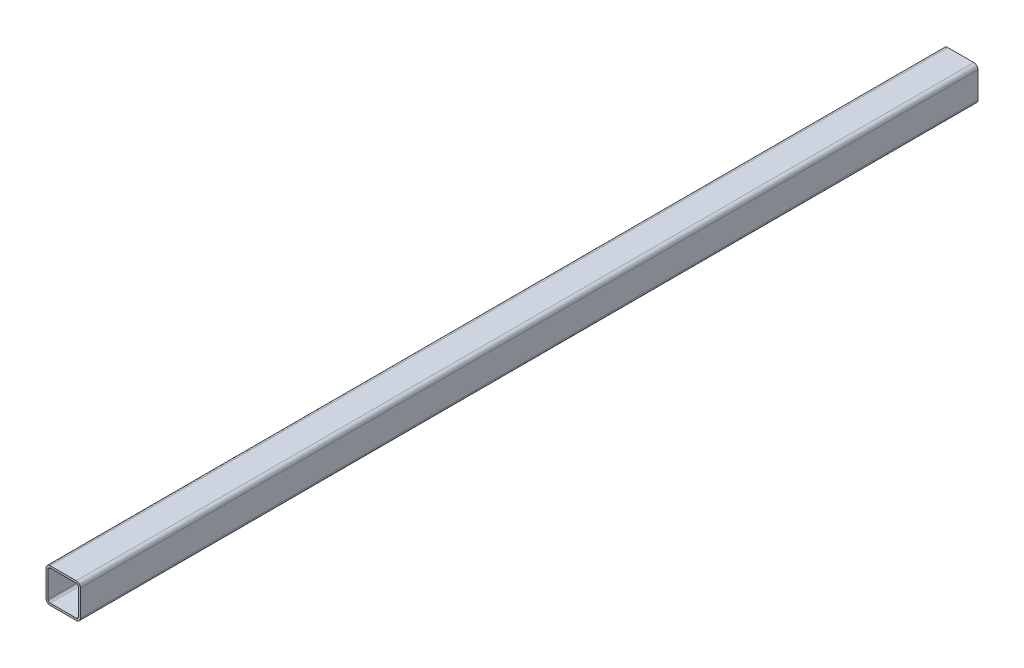
SolidWorks part; units mm, degrees
material "Q235B"
ref_plane "前视基准面" through (0, 0, 0) normal (0, 0, 1) x (1, 0, 0)
ref_plane "上视基准面" through (0, 0, 0) normal (0, 1, 0) x (1, 0, 0)
ref_plane "右视基准面" through (0, 0, 0) normal (1, 0, 0) x (0, 0, -1)
other "Configuration Table"
sketch "草图1" plane through (0, 0, 0) normal (1, 0, 0) x (0, 0, -1)
  line L0 (-652.5, 0) -> (652.5, 0)
other "Gb／6728-1986方形空心型钢 050 X 50 X 3(1)"
ref_plane "基准面1" through (0, 0, 652.5) normal (0, 0, -1) x (0, 1, 0)
sketch "Sketch1" plane through (0, 0, 652.5) normal (0, 0, -1) x (0, 1, 0)
  line L0 (-19, -22) -> (19, -22)
  line L1 (-22, -19) -> (-22, 19)
  line L2 (19, 22) -> (-19, 22)
  line L3 (22, 19) -> (22, -19)
  line L4 (-19, -25) -> (19, -25)
  line L5 (-25, -19) -> (-25, 19)
  line L6 (19, 25) -> (-19, 25)
  line L7 (25, 19) -> (25, -19)
  arc A0 (25, 19) -> (19, 25) centre (19, 19) ccw
  arc A1 (19, -25) -> (25, -19) centre (19, -19) ccw
  arc A2 (-25, -19) -> (-19, -25) centre (-19, -19) ccw
  arc A3 (-19, 25) -> (-25, 19) centre (-19, 19) ccw
  arc A4 (-19, 22) -> (-22, 19) centre (-19, 19) ccw
  arc A5 (22, 19) -> (19, 22) centre (19, 19) ccw
  arc A6 (19, -22) -> (22, -19) centre (19, -19) ccw
  arc A7 (-22, -19) -> (-19, -22) centre (-19, -19) ccw
  point P0 (-25, 0)
  point P1 (25, 0)
  point P2 (0, 25)
  point P3 (0, -25)
  point P4 (0, 0)
  point P5 (-25, -25)
  point P6 (25, -25)
  point P7 (25, 25)
  point P8 (-25, 25)
  point P33 (0, 0)
  dimension "D1" = 6
  dimension "Thickness" = 3
  dimension "V_leg" = 50
equation "\"D2@草图1\"=\"D1@草图1\"/2"
